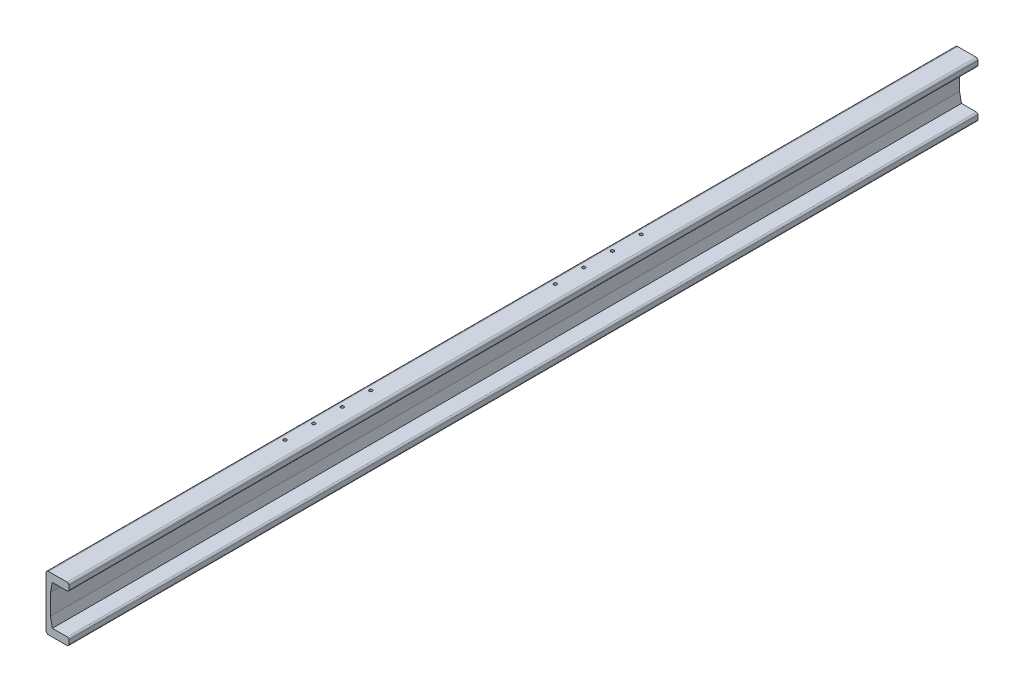
from build123d import *

# Parameters (mm, degrees)
BOSS_EXTRUDE1_DEPTH   = 1430
M6_TAPPED_HOLE1_D     = 5
M6_TAPPED_HOLE1_DEPTH = 15
M6_TAPPED_HOLE1_TIP   = 1.502151548


with BuildPart() as part:
    # Sketch1 → Boss-Extrude1 (new body)
    with BuildSketch(Plane.XY):
        with BuildLine():
            Line((-3, 0), (-32, 0))
            ThreePointArc((-32, 0), (-34.828427125, -1.171572875), (-36, -4))
            Line((-36, -4), (-36, -82.5))
            ThreePointArc((-36, -82.5), (-34.828427125, -85.328427125), (-32, -86.5))
            Line((-32, -86.5), (-3, -86.5))
            ThreePointArc((-3, -86.5), (-0.878679656, -85.621320344), (0, -83.5))
            Line((0, -83.5), (0, -77))
            ThreePointArc((0, -77), (-0.732233047, -75.232233047), (-2.5, -74.5))
            Line((-2.5, -74.5), (-26, -74.5))
            Line((-26, -74.5), (-29, -59.5))
            Line((-29, -59.5), (-29, -27))
            Line((-29, -27), (-26, -12))
            Line((-26, -12), (-2.5, -12))
            ThreePointArc((-2.5, -12), (-0.732233047, -11.267766953), (0, -9.5))
            Line((0, -9.5), (0, -3))
            ThreePointArc((0, -3), (-0.878679656, -0.878679656), (-3, 0))
        make_face()
    extrude(amount=BOSS_EXTRUDE1_DEPTH)

    # M6 Tapped Hole1
    with Locations(Plane(origin=(0, 0, 0), x_dir=(1, 0, 0), z_dir=(0, 1, 0))):
        with Locations((-25, -505), (-25, -550), (-25, -595), (-25, -640), (-25, -930), (-25, -975), (-25, -1020), (-25, -1065)):
            Hole(M6_TAPPED_HOLE1_D / 2, depth=M6_TAPPED_HOLE1_DEPTH)
            with Locations((0, 0, -(M6_TAPPED_HOLE1_DEPTH + M6_TAPPED_HOLE1_TIP / 2))):  # 118° drill point
                Cone(0, M6_TAPPED_HOLE1_D / 2, M6_TAPPED_HOLE1_TIP, mode=Mode.SUBTRACT)


solid = part.part
